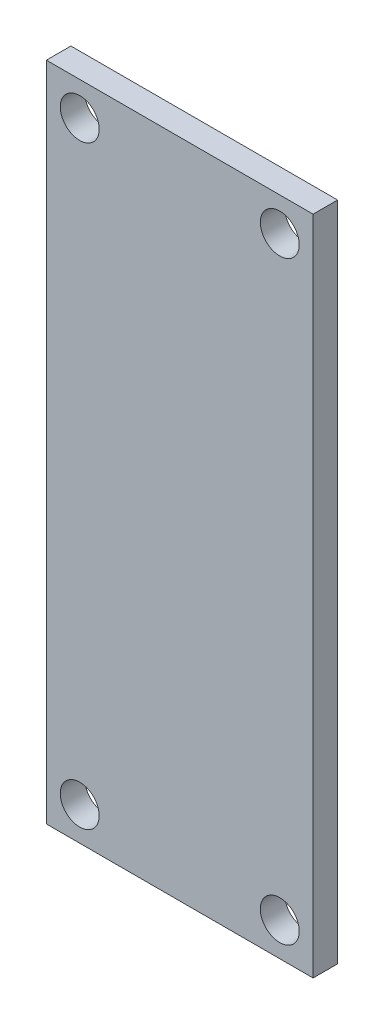
SolidWorks part; units mm, degrees
material "普通碳钢"
ref_plane "Front Plane" through (0, 0, 0) normal (0, 0, 1) x (1, 0, 0)
ref_plane "Top Plane" through (0, 0, 0) normal (0, 1, 0) x (1, 0, 0)
ref_plane "Right Plane" through (0, 0, 0) normal (1, 0, 0) x (0, 0, -1)
sketch "Sketch1" plane through (0, 0, 0) normal (0, 0, 1) x (1, 0, 0)
  line L0 (57.15, 211.8089) -> (57.15, -203.7098) construction
  line L1 (-76.2, 188.975) -> (76.2, 188.975)
  line L2 (-76.2, 188.975) -> (-76.2, -188.975)
  line L3 (-76.2, -188.975) -> (76.2, -188.975)
  line L4 (76.2, 188.975) -> (76.2, -188.975)
  line L5 (-76.2, 188.975) -> (76.2, -188.975) construction
  line L6 (-76.2, -188.975) -> (76.2, 188.975) construction
  line L7 (-57.15, 211.8089) -> (-57.15, -203.7098) construction
  line L8 (-95.7963, 169.8625) -> (88.8378, 169.8625) construction
  line L9 (-95.7963, -169.8625) -> (88.8378, -169.8625) construction
  line L10 (0, 0) -> (0, -208.0452) construction
  line L11 (0, 0) -> (88.8378, 0) construction
  circle A0 centre (-57.15, 169.8625) radius 11.125
  circle A1 centre (57.15, 169.8625) radius 11.125
  circle A2 centre (57.15, -169.8625) radius 11.125
  circle A3 centre (-57.15, -169.8625) radius 11.125
  point P0 (0, 0)
  dimension "D5" = 22.25
  dimension "D1" = 377.95
  dimension "D2" = 152.4
  dimension "D3" = 339.725
  dimension "D4" = 114.3
extrude "Boss-Extrude1" add sketch "Sketch1" along normal blind 14
